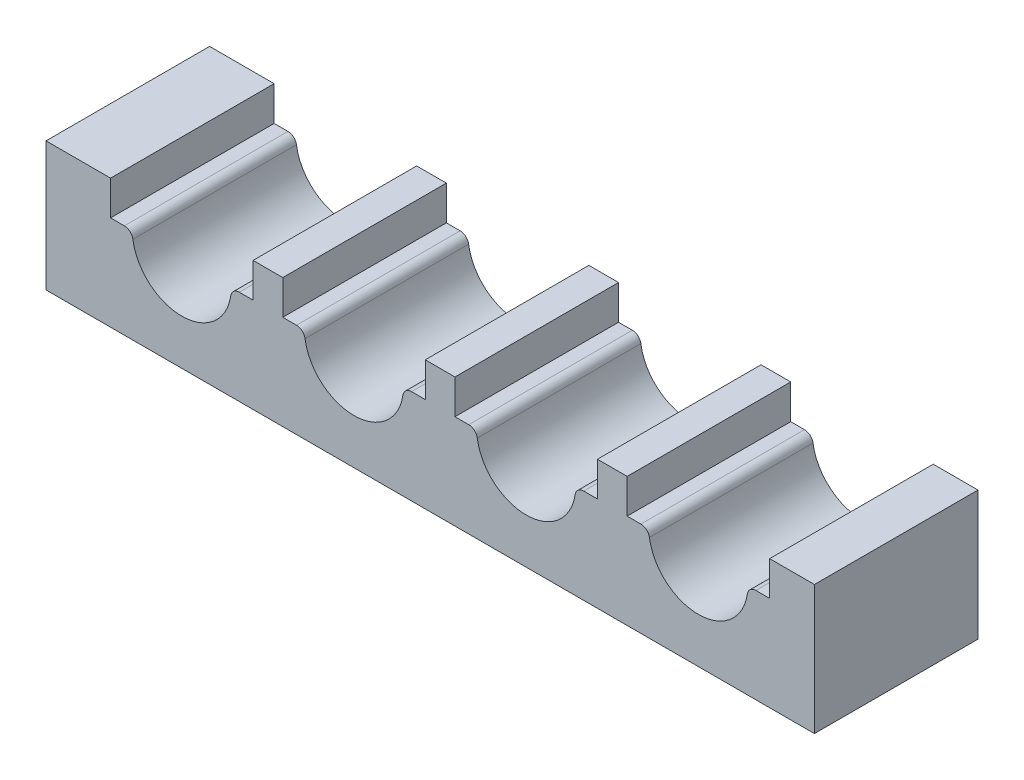
from build123d import *

# Parameters (mm, degrees)
SKETCH1_W              = 357
SKETCH1_H              = 60
BOSS_EXTRUDE1_DEPTH    = 76
SKETCH2_W              = 66.2
SKETCH2_H              = 36
CUT_EXTRUDE1_DEPTH     = 197.311614532
SKETCH3_R              = 23
CUT_EXTRUDE2_DEPTH     = 197.311614532
FILLET1_R              = 4
LPATTERN1_COUNT        = 4
LPATTERN1_PITCH        = 80
FILLET1_OF_LPATTERN1_R = 4


with BuildPart() as part:
    # Sketch1 → Boss-Extrude1 (new body)
    with BuildSketch(Plane.XY):
        Rectangle(SKETCH1_W, SKETCH1_H)
    extrude(amount=BOSS_EXTRUDE1_DEPTH)

    # Sketch2 → Cut-Extrude1 (cut, through all)
    with BuildSketch(Plane.XY.offset(76)):
        with Locations((-115.4, 32)):
            Rectangle(SKETCH2_W, SKETCH2_H)
    cut_extrude1 = extrude(amount=-CUT_EXTRUDE1_DEPTH, mode=Mode.SUBTRACT)

    # Sketch3 → Cut-Extrude2 (cut, through all)
    with BuildSketch(Plane.XY.offset(76)):
        with Locations((-115.4, 14)):
            Circle(SKETCH3_R)
    cut_extrude2 = extrude(amount=-CUT_EXTRUDE2_DEPTH, mode=Mode.SUBTRACT)

    # Fillet1
    fillet1_edges = [part.edges().sort_by_distance(p)[0] for p in [
        (-138.4, 14, 38),
        (-92.4, 14, 38),
    ]]
    fillet(fillet1_edges, radius=FILLET1_R)

    # LPattern1: Cut-Extrude1, Cut-Extrude2 ×4
    with Locations(*[(i * LPATTERN1_PITCH, 0, 0) for i in range(1, LPATTERN1_COUNT)]):
        add(cut_extrude1, mode=Mode.SUBTRACT)
        add(cut_extrude2, mode=Mode.SUBTRACT)

    # Fillet1 of LPattern1
    fillet1_of_lpattern1_edges = [part.edges().sort_by_distance(p)[0] for p in [
        (-58.4, 14, 38),
        (-12.4, 14, 38),
        (21.6, 14, 38),
        (67.6, 14, 38),
        (101.6, 14, 38),
        (147.6, 14, 38),
    ]]
    fillet(fillet1_of_lpattern1_edges, radius=FILLET1_OF_LPATTERN1_R)


solid = part.part
